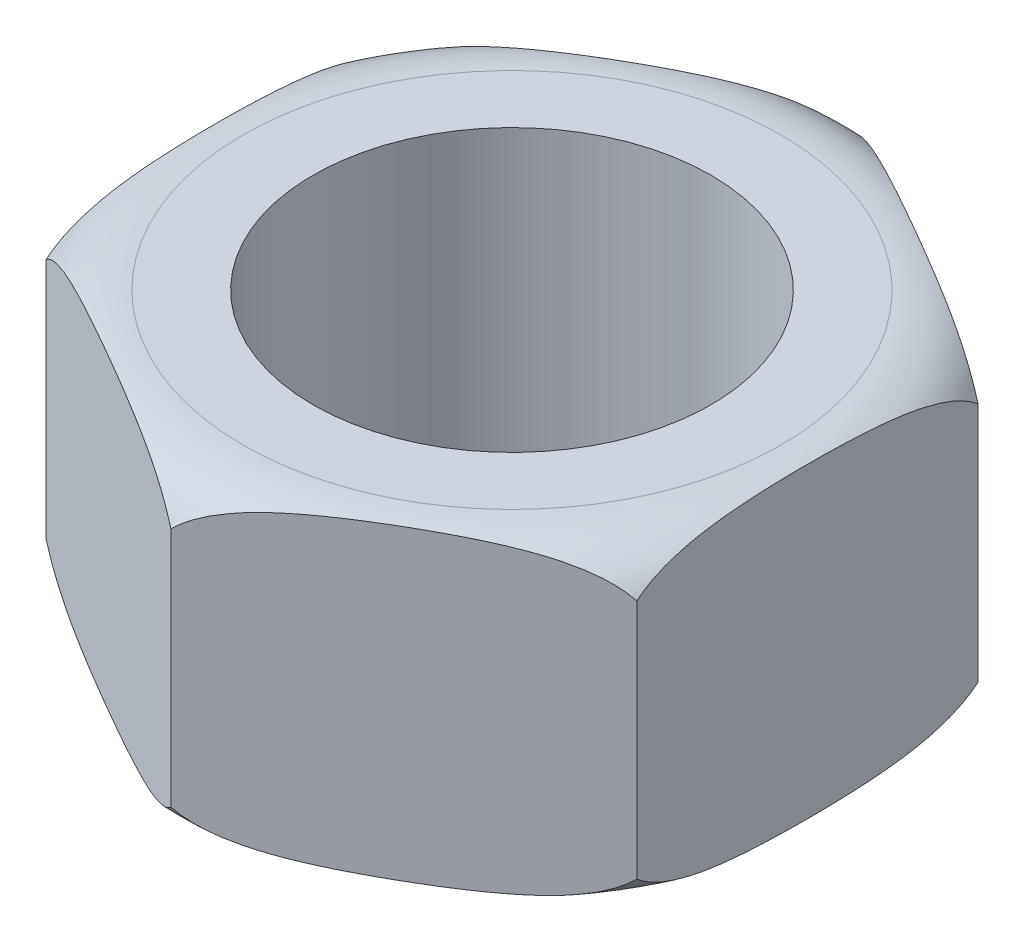
SolidWorks part; units mm, degrees
ref_plane "Front Plane" through (0, 0, 0) normal (0, 0, 1) x (1, 0, 0)
ref_plane "Top Plane" through (0, 0, 0) normal (0, 1, 0) x (1, 0, 0)
ref_plane "Right Plane" through (0, 0, 0) normal (1, 0, 0) x (0, 0, -1)
sketch "Sketch 1" plane through (0, 0, 0) normal (0, 1, 0) x (1, 0, 0)
  line L1 (0, 28.2902) -> (-24.5, 14.1451)
  line L2 (-24.5, 14.1451) -> (-24.5, -14.1451)
  line L3 (-24.5, -14.1451) -> (0, -28.2902)
  line L4 (0, -28.2902) -> (24.5, -14.1451)
  line L5 (24.5, -14.1451) -> (24.5, 14.1451)
  line L6 (24.5, 14.1451) -> (0, 28.2902)
  circle A0 centre (0, 0) radius 16.5
  circle A1 centre (0, 0) radius 24.5 construction
  dimension "D1" = 33
  dimension "D2" = 49
extrude "Boss-Extrude 1" add sketch "Sketch 1" along normal mid plane 26
sketch "Sketch 2" plane through (0, 0, 0) normal (1, 0, 0) x (0, 0, -1)
  line L0 (0, 20.7202) -> (0, -24.738) construction
  line L1 (-40.7516, 0) -> (40.6368, 0) construction
  line L2 (-28.2902, 13) -> (-28.2902, -13) construction
  line L3 (-14.1451, 13) -> (14.1451, 13) construction
  line L4 (-22.2902, 13) -> (-28.2902, 13)
  line L5 (-28.2902, 13) -> (-28.2902, 10)
  line L8 (-28.2902, -13) -> (-28.2902, -10)
  line L9 (-22.2902, -13) -> (-28.2902, -13)
  spline S0 degree 3 poles (-28.2902, 10) (-27.0287, 12.129) (-24.7115, 13) (-22.2902, 13) knots 0 0 0 0 1 1 1 1
  spline S1 degree 3 poles (-28.2902, -10) (-27.0287, -12.129) (-24.7115, -13) (-22.2902, -13) knots 0 0 0 0 1 1 1 1
  dimension "D1" = 2
  dimension "D2" = 3
  dimension "D3" = 6
  dimension "D4" = 1
revolve "Cut-Revolve 1" cut sketch "Sketch 2" angle 360 about L0
